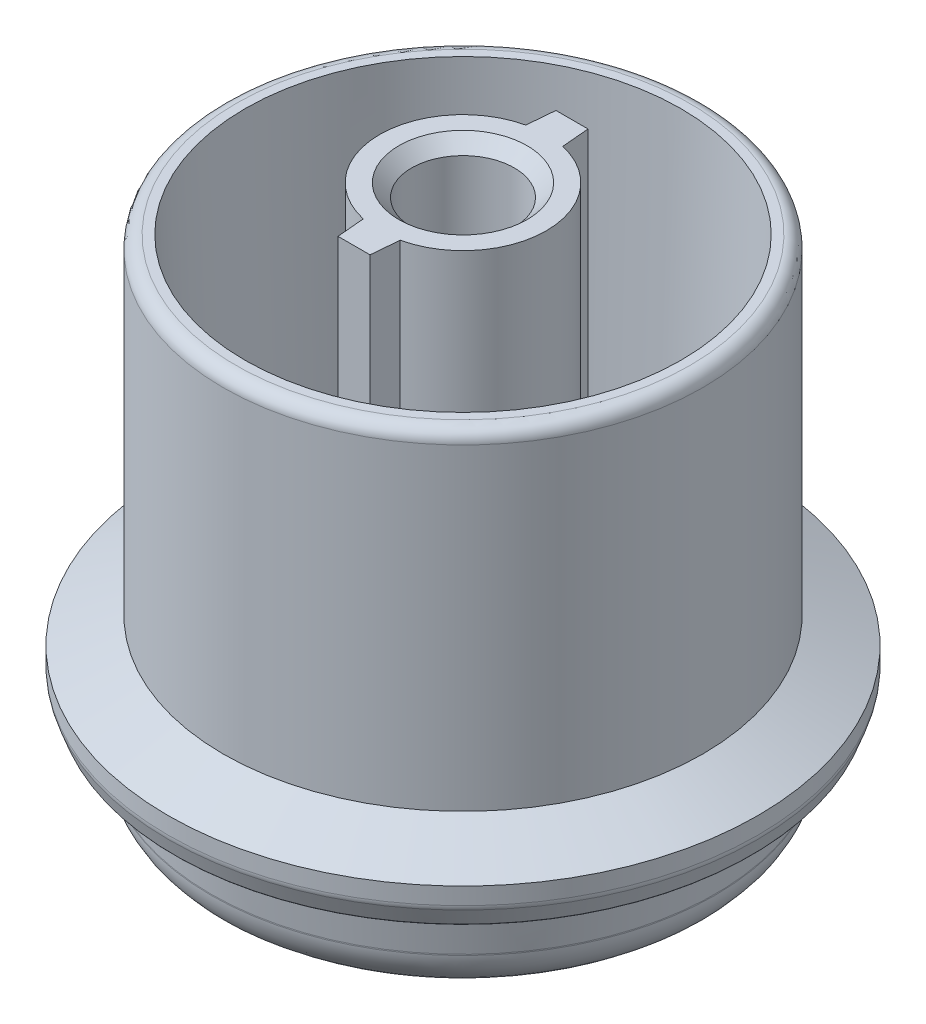
from build123d import *

# Parameters (mm, degrees)
CHAMFER1_SIZE       = 3
CHAMFER1_SIZE2      = 1.091910703
SKETCH4_R           = 13
BOSS_EXTRUDE1_DEPTH = 75
BOSS_EXTRUDE2_DEPTH = 75
CIRPATTERN1_COUNT   = 2
FILLET1_R           = 2
FILLET2_R           = 2
SKETCH6_W           = 10
SKETCH6_H           = 32
SKETCH7_R           = 8
CUT_EXTRUDE1_DEPTH  = 30
SKETCH8_R           = 3
CUT_EXTRUDE2_DEPTH  = 30
CHAMFER2_SIZE       = 2
SKETCH9_R           = 10
CUT_EXTRUDE3_DEPTH  = 10
CHAMFER3_SIZE       = 1
FILLET3_R           = 7
FILLET4_R           = 2
FILLET5_R           = 0.2
FILLET6_R           = 1.25
FILLET7_R           = 0.2


with BuildPart() as part:
    # Sketch2 → Revolve1 (revolve)
    with BuildSketch(Plane.XY, mode=Mode.PRIVATE) as revolve1_sk:
        Polygon((0, 0), (40, 0), (40, 14.5), (46, 14.5), (46, 20.5), (37.4, 24.51024586), (37.4, 76), (0, 76), align=None)
    revolve(revolve1_sk.sketch.rotate(Axis((0, 76, 0), (0, -1, 0)), 180), axis=Axis((0, 76, 0), (0, -1, 0)))

    # Chamfer1
    chamfer1_edges = [part.edges().sort_by_distance(p)[0] for p in [
        (46, 14.5, 0),
    ]]
    chamfer1_side = [part.faces().sort_by_distance(p)[0] for p in [
        (46, 17.5, 0),
    ]]
    chamfer(chamfer1_edges, length=CHAMFER1_SIZE, length2=CHAMFER1_SIZE2, reference=chamfer1_side[0])

    # Sketch3 → Cut-Revolve1 (revolve, cut)
    with BuildSketch(Plane.XY, mode=Mode.PRIVATE) as cut_revolve1_sk:
        Polygon((34, 76), (0, 76), (0, 8), (31.625387675, 8), align=None)
    revolve(cut_revolve1_sk.sketch.rotate(Axis((0, 134.916718262, 0), (0, -1, 0)), 90), axis=Axis((0, 134.916718262, 0), (0, -1, 0)), mode=Mode.SUBTRACT)

    # Sketch4 → Boss-Extrude1 (add)
    with BuildSketch(Plane(origin=(0, 8, 0), x_dir=(1, 0, 0), z_dir=(0, 1, 0))):
        with Locations(Location((0, 0, 0), (0, 0, 270))):
            Circle(SKETCH4_R)
    extrude(amount=BOSS_EXTRUDE1_DEPTH)

    # Sketch5 → Boss-Extrude2 (add)
    with BuildSketch(Plane(origin=(0, 8, 0), x_dir=(1, 0, 0), z_dir=(0, 1, 0))):
        with BuildLine():
            Line((-2.5, 17), (-2.878179843, 12.67738462))
            ThreePointArc((-2.878179843, 12.67738462), (0, 13), (2.878179843, 12.67738462))
            Line((2.878179843, 12.67738462), (2.5, 17))
            Line((2.5, 17), (-2.5, 17))
        make_face()
    boss_extrude2 = extrude(amount=BOSS_EXTRUDE2_DEPTH)

    # CirPattern1: Boss-Extrude2 ×2 about axis
    cirpattern1_axis = Axis((0, 0, 0), (0, 1, 0))
    for i in range(1, CIRPATTERN1_COUNT):
        add(boss_extrude2.rotate(cirpattern1_axis, i * 360 / CIRPATTERN1_COUNT))

    # Fillet1
    fillet1_edges = [part.edges().sort_by_distance(p)[0] for p in [
        (0, 8, -31.625387675),
    ]]
    fillet(fillet1_edges, radius=FILLET1_R)

    # Fillet2
    fillet2_edges = [part.edges().sort_by_distance(p)[0] for p in [
        (37.4, 76, 0),
    ]]
    fillet(fillet2_edges, radius=FILLET2_R)

    # Sketch6 → Cut-Revolve2 (revolve, cut)
    with BuildSketch(Plane(origin=(0, 0, 0), x_dir=(0, 0, -1), z_dir=(1, 0, 0)), mode=Mode.PRIVATE) as cut_revolve2_sk:
        with Locations((5, 42)):
            Rectangle(SKETCH6_W, SKETCH6_H)
    revolve(cut_revolve2_sk.sketch.rotate(Axis((0, 140.488845923, 0), (0, -1, 0)), 90), axis=Axis((0, 140.488845923, 0), (0, -1, 0)), mode=Mode.SUBTRACT)

    # Sketch7 → Cut-Extrude1 (cut)
    with BuildSketch(Plane(origin=(0, 83, 0), x_dir=(1, 0, 0), z_dir=(0, 1, 0))):
        with Locations(Location((0, 0, 0), (0, 0, 270))):
            Circle(SKETCH7_R)
    extrude(amount=-CUT_EXTRUDE1_DEPTH, mode=Mode.SUBTRACT)

    # Sketch8 → Cut-Extrude2 (cut)
    with BuildSketch(Plane.XZ):
        with Locations((-20, 0)):
            Circle(SKETCH8_R)
        with Locations((20, 0)):
            Circle(SKETCH8_R)
    extrude(amount=-CUT_EXTRUDE2_DEPTH, mode=Mode.SUBTRACT)

    # Chamfer2
    chamfer2_edges = [part.edges().sort_by_distance(p)[0] for p in [
        (0, 83, -8),
    ]]
    chamfer(chamfer2_edges, length=CHAMFER2_SIZE)

    # Sketch9 → Cut-Extrude3 (cut)
    with BuildSketch(Plane.XZ):
        with Locations(Location((0, 0, 0), (0, 0, 90))):
            Circle(SKETCH9_R)
    extrude(amount=-CUT_EXTRUDE3_DEPTH, mode=Mode.SUBTRACT)

    # Chamfer3
    chamfer3_edges = [part.edges().sort_by_distance(p)[0] for p in [
        (0, 0, -10),
    ]]
    chamfer(chamfer3_edges, length=CHAMFER3_SIZE)

    # Sketch10 → Cut-Revolve3 (revolve, cut)
    with BuildSketch(Plane.XY, mode=Mode.PRIVATE) as cut_revolve3_sk:
        with BuildLine():
            Line((-43.4, 14.5), (-43.4, 18))
            Line((-43.4, 18), (-40.65, 18))
            ThreePointArc((-40.65, 18), (-39.658308325, 17.510951786), (-39.442592717, 16.426476194))
            Line((-39.442592717, 16.426476194), (-39.783754868, 15.153241714))
            ThreePointArc((-39.783754868, 15.153241714), (-39.773321328, 15.020226176), (-39.681554213, 14.923371704))
            ThreePointArc((-39.681554213, 14.923371704), (-39.319426642, 14.136232165), (-40, 13.6))
            Line((-40, 13.6), (-39.335, 6.57))
            Line((-39.335, 6.57), (-38.760199481, 0))
            Line((-38.760199481, 0), (-43.4, 0))
            Line((-43.4, 0), (-43.4, 14.5))
        make_face()
    revolve(cut_revolve3_sk.sketch.rotate(Axis((0, 143.968242968, 0), (0, -1, 0)), 270), axis=Axis((0, 143.968242968, 0), (0, -1, 0)), mode=Mode.SUBTRACT)

    # Fillet3
    fillet3_edges = [part.edges().sort_by_distance(p)[0] for p in [
        (0, 0, -38.760199481),
    ]]
    fillet(fillet3_edges, radius=FILLET3_R)

    # Fillet4
    fillet4_edges = [part.edges().sort_by_distance(p)[0] for p in [
        (46, 17.5, 0),
    ]]
    fillet(fillet4_edges, radius=FILLET4_R)

    # Fillet5
    fillet5_edges = [part.edges().sort_by_distance(p)[0] for p in [
        (0, 14.5, -43.4),
        (44.908089297, 14.5, 0),
    ]]
    fillet(fillet5_edges, radius=FILLET5_R)

    # Fillet6
    fillet6_edges = [part.edges().sort_by_distance(p)[0] for p in [
        (0, 18, -43.4),
    ]]
    fillet(fillet6_edges, radius=FILLET6_R)

    # Fillet7
    fillet7_edges = [part.edges().sort_by_distance(p)[0] for p in [
        (0, 13.6, -40),
    ]]
    fillet(fillet7_edges, radius=FILLET7_R)


solid = part.part
